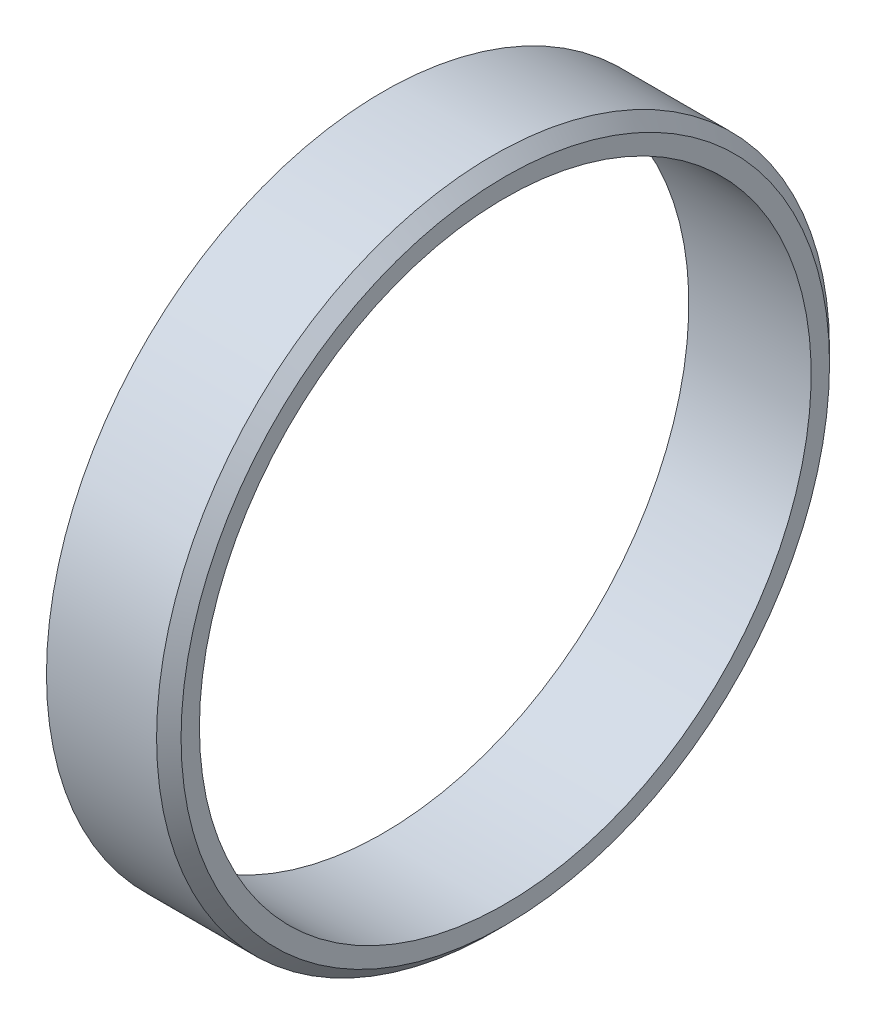
from build123d import *

# Parameters (mm, degrees)
SKETCH_1_W     = 10
SKETCH_1_H     = 2.5
CHAMFER_1_SIZE = 1


with BuildPart() as part:
    # 草图1 → 旋转1 (revolve)
    with BuildSketch(Plane(origin=(0, 0, 0), x_dir=(1, 0, 0), z_dir=(0, 1, 0)), mode=Mode.PRIVATE) as revolve_1_sk:
        with Locations((5, 26.25)):
            Rectangle(SKETCH_1_W, SKETCH_1_H)
    revolve(revolve_1_sk.sketch.rotate(Axis((-308.212798969, 0, 0), (1, 0, 0)), 180), axis=Axis((-308.212798969, 0, 0), (1, 0, 0)))

    # 倒角1
    chamfer_1_edges = [part.edges().sort_by_distance(p)[0] for p in [
        (10, 0, -27.5),
    ]]
    chamfer(chamfer_1_edges, length=CHAMFER_1_SIZE)


solid = part.part
